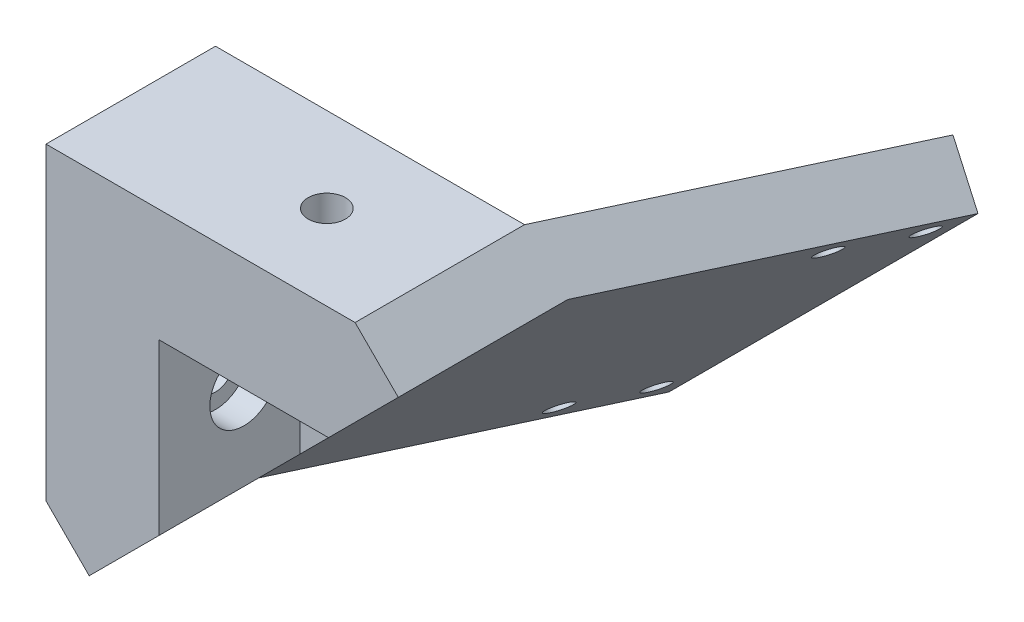
SolidWorks part; units mm, degrees
ref_plane "前视基准面" through (0, 0, 0) normal (0, 0, 1) x (1, 0, 0)
ref_plane "上视基准面" through (0, 0, 0) normal (0, 1, 0) x (1, 0, 0)
ref_plane "右视基准面" through (0, 0, 0) normal (1, 0, 0) x (0, 0, -1)
sketch "草图1" plane through (0, 0, 0) normal (0, 0, 1) x (1, 0, 0)
  line L0 (0, 0) -> (70, 0)
  line L1 (70, 0) -> (0, -70)
  line L2 (0, -70) -> (0, 0)
  dimension "D1" = 70
extrude "凸台-拉伸1" add sketch "草图1" along normal mid plane 30
sketch "草图4" plane through (0, 0, 15) normal (0, 0, 1) x (1, 0, 0)
  line L0 (0, 0) -> (35, -35) construction
  line L1 (0, -70) -> (70, 0) construction
ref_plane "基准面2" through (0, 0, 0) normal (-0.7071, -0.7071, 0) x (0.7071, -0.7071, 0)
sketch "草图5" plane through (0, 0, 0) normal (-0.7071, -0.7071, 0) x (0.7071, -0.7071, 0)
  line L0 (49.4975, -15) -> (65.854, -76.0435)
  line L3 (49.4975, 15) -> (49.4975, -15) construction
  line L4 (38.682, -15) -> (55.763, -78.7474)
  line L5 (0, -15) -> (49.4975, -15) construction
  line L6 (55.763, -78.7474) -> (65.854, -76.0435)
  line L7 (0, -15) -> (49.4975, -15)
  dimension "D1" = 165
extrude "凸台-拉伸2" add sketch "草图5" along normal up to vertex (49.4975 mm away) and the other way up to vertex (49.4975 mm away) contours L7 L4 L6 L0 up to point (0, -70, -15) other way up to point (70, 0, -15)
sketch "草图7" plane through (0, 0, 15) normal (0, 0, 1) x (1, 0, 0)
  line L0 (54.7046, 0) -> (107.7406, -53.0361)
  line L1 (0, -54.7046) -> (47.1689, -101.8735)
  line L2 (70, 0) -> (81.5658, -11.5658) construction
  line L3 (11.5658, -81.5658) -> (81.5658, -11.5658) construction
  line L4 (81.5658, -11.5658) -> (70, 0) construction
  line L5 (70, 0) -> (0, -70) construction
  line L6 (0, -70) -> (11.5658, -81.5658) construction
  line L7 (0, -70) -> (0, -54.7046) construction
  line L8 (0, -54.7046) -> (-7.6477, -62.3523) construction
  line L9 (-7.6477, -62.3523) -> (0, -70) construction
  line L10 (54.7046, 0) -> (70, 0) construction
  line L11 (70, 0) -> (62.3523, 7.6477) construction
  line L12 (62.3523, 7.6477) -> (54.7046, 0) construction
  line L13 (11.5658, -81.5658) -> (81.5658, -11.5658)
  line L14 (81.5658, -11.5658) -> (70, 0)
  line L15 (70, 0) -> (0, -70)
  line L16 (0, -70) -> (11.5658, -81.5658)
  line L17 (0, -70) -> (0, -54.7046)
  line L18 (0, -54.7046) -> (-7.6477, -62.3523)
  line L19 (-7.6477, -62.3523) -> (0, -70)
  line L20 (54.7046, 0) -> (70, 0)
  line L21 (70, 0) -> (62.3523, 7.6477)
  line L22 (62.3523, 7.6477) -> (54.7046, 0)
  line M2 (0, 0) -> (0, -70)
  line M3 (0, -70) -> (70, 0)
  line M4 (70, 0) -> (0, 0)
extrude "切除-拉伸3" cut sketch "草图7" against normal blind 113 contours L0 M4 M3 | L21 L22 M4 | L13 L14 L0 M3 | L16 L13 L1 M3 | L1 M2 M3 | L18 L19 M2
sketch "草图8" plane through (0, 0, 0) normal (0, 1, 0) x (1, 0, 0)
  line L0 (14.7046, 0) -> (54.7046, 0) construction
  line L1 (54.7046, 15) -> (54.7046, -15) construction
  circle A0 centre (34.7046, 0) radius 3.3
  dimension "D1" = 6.6
  dimension "D2" = 40
extrude "切除-拉伸4" cut sketch "草图8" against normal blind 113
sketch "草图9" plane through (0, 0, 0) normal (0, 1, 0) x (1, 0, 0)
  circle A0 centre (34.7046, 0) radius 6
  dimension "D1" = 12
extrude "切除-拉伸5" cut sketch "草图9" against normal blind 113 from offset 15 offset against normal yes
sketch "草图10" plane through (0, 0, 15) normal (0, 0, 1) x (1, 0, 0)
  line L2 (20, -54.7046) -> (12.6477, -57.3523)
  line L3 (7.6477, -62.3523) -> (62.3523, -7.6477) construction
  line L4 (20, -20) -> (20, -54.7046)
  line L5 (54.7046, -20) -> (20, -20)
  line L6 (20, -20) -> (20, -54.7046)
  line L7 (54.7046, -20) -> (20, -20)
  line L8 (54.7046, -20) -> (47.3523, -22.6477)
  line L9 (7.6477, -62.3523) -> (62.3523, -7.6477) construction
  line L10 (7.6477, -62.3523) -> (62.3523, -7.6477)
  line M3 (7.6477, -62.3523) -> (62.3523, -7.6477)
  dimension "D1" = 20
extrude "切除-拉伸6" cut sketch "草图10" against normal blind 25 contours L8 L7 L6 L2 M3
mirror "镜向2" about plane through (0, 0, 0) normal (-0.7071, -0.7071, 0) of "切除-拉伸4", "切除-拉伸5"
sketch "草图11" plane through (30.0038, -30.0038, 11.3696) normal (0.683, -0.683, 0.2588) x (0.183, -0.183, -0.9659)
  line L4 (70.4967, 33.682) -> (70.4967, -33.682) construction
  line L8 (85.4967, 33.682) -> (32.2998, 33.682)
  line L9 (32.2998, 33.682) -> (32.2998, -33.682)
  line L10 (32.2998, -33.682) -> (85.4967, -33.682)
  line L11 (85.4967, -33.682) -> (85.4967, 33.682)
  line L12 (85.4967, 33.682) -> (70.4967, 33.682) construction
  line L14 (70.4967, -33.682) -> (85.4967, -33.682) construction
  line L15 (85.4967, -33.682) -> (85.4967, 33.682) construction
  circle A0 centre (70.4967, 33.682) radius 2.2
  circle A1 centre (85.4967, 33.682) radius 2.2
  circle A2 centre (85.4967, -33.682) radius 2.2
  circle A3 centre (70.4967, -33.682) radius 2.2
  dimension "D3" = 4.4
  dimension "D2" = 15
  dimension "D1" = 5
extrude "切除-拉伸7" cut sketch "草图11" against normal blind 30
